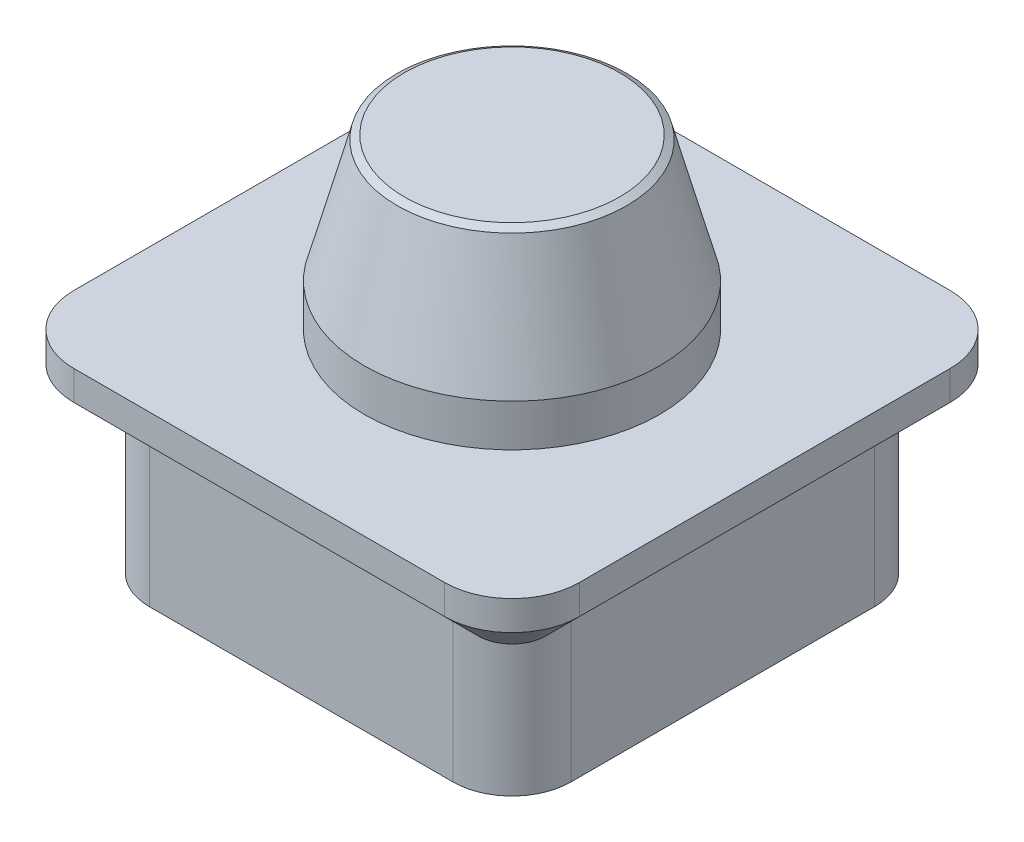
from build123d import *

# Parameters (mm, degrees)
CHAMFER1_SIZE       = 1
CHAMFER1_SIZE2      = 1.414213562
BOSS_EXTRUDE1_DEPTH = 15
BOSS_EXTRUDE2_DEPTH = 35
CHAMFER2_SIZE       = 8


with BuildPart() as part:
    # Sketch1 → Revolve1 (revolve)
    with BuildSketch(Plane.XY, mode=Mode.PRIVATE) as revolve1_sk:
        Polygon((0, 0), (35, 0), (35, 10), (26.961524227, 40), (0, 40), align=None)
    revolve(revolve1_sk.sketch.rotate(Axis((0, 40, 0), (0, -1, 0)), 180), axis=Axis((0, 40, 0), (0, -1, 0)))

    # Chamfer1
    chamfer1_edges = [part.edges().sort_by_distance(p)[0] for p in [
        (26.961524227, 40, 0),
    ]]
    chamfer1_side = [part.faces().sort_by_distance(p)[0] for p in [
        (30.980762114, 25, 0),
    ]]
    chamfer(chamfer1_edges, length=CHAMFER1_SIZE, length2=CHAMFER1_SIZE2, reference=chamfer1_side[0])

    # Sketch2 → Boss-Extrude1 (add)
    with BuildSketch(Plane.XZ):
        with BuildLine():
            Line((44, -60), (-44, -60))
            ThreePointArc((-44, -60), (-55.313708499, -55.313708499), (-60, -44))
            Line((-60, -44), (-60, 44))
            ThreePointArc((-60, 44), (-55.313708499, 55.313708499), (-44, 60))
            Line((-44, 60), (44, 60))
            ThreePointArc((44, 60), (55.313708499, 55.313708499), (60, 44))
            Line((60, 44), (60, -44))
            ThreePointArc((60, -44), (55.313708499, -55.313708499), (44, -60))
        make_face()
    extrude(amount=BOSS_EXTRUDE1_DEPTH)

    # Sketch3 → Boss-Extrude2 (add)
    with BuildSketch(Plane.XZ.offset(15)):
        with BuildLine():
            Line((36, -50), (-36, -50))
            ThreePointArc((-36, -50), (-45.899494937, -45.899494937), (-50, -36))
            Line((-50, -36), (-50, 36))
            ThreePointArc((-50, 36), (-45.899494937, 45.899494937), (-36, 50))
            Line((-36, 50), (36, 50))
            ThreePointArc((36, 50), (45.899494937, 45.899494937), (50, 36))
            Line((50, 36), (50, -36))
            ThreePointArc((50, -36), (45.899494937, -45.899494937), (36, -50))
        make_face()
    extrude(amount=BOSS_EXTRUDE2_DEPTH)

    # Chamfer2
    chamfer2_edges = [part.edges().sort_by_distance(p)[0] for p in [
        (-55.313708499, -15, -55.313708499),
        (0, -15, -60),
        (55.313708499, -15, -55.313708499),
        (60, -15, 0),
        (55.313708499, -15, 55.313708499),
        (0, -15, 60),
        (-55.313708499, -15, 55.313708499),
        (-60, -15, 0),
    ]]
    chamfer(chamfer2_edges, length=CHAMFER2_SIZE)


solid = part.part
